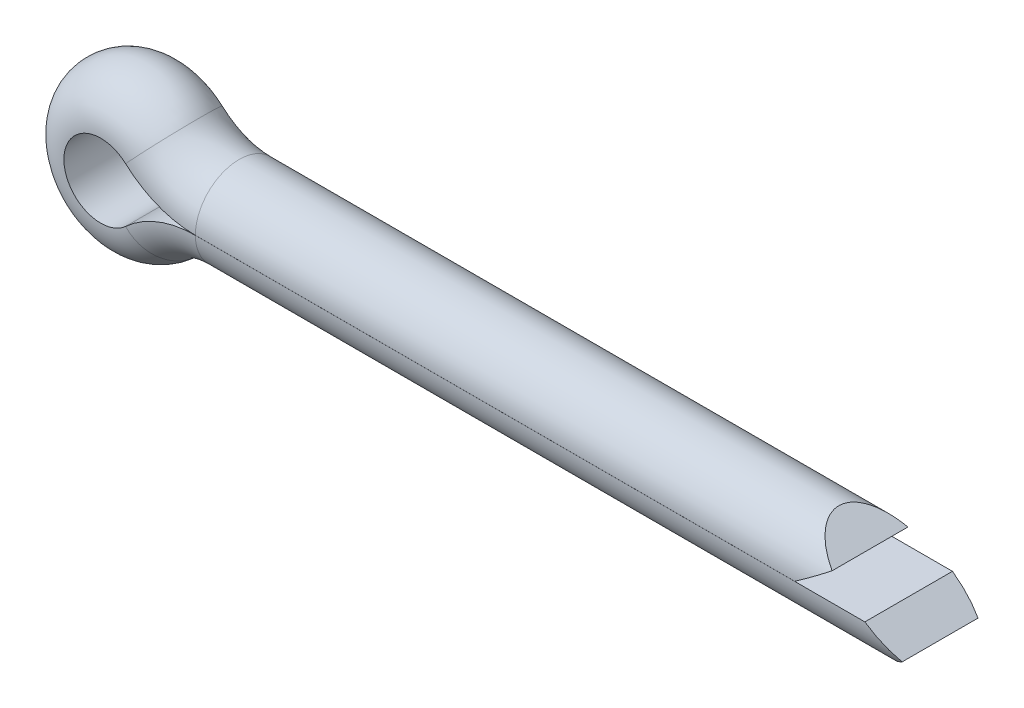
from build123d import *

# Parameters (mm, degrees)
CONECUT_DEPTH      = 41.341170006
CONECUT_DEPTH_BACK = 41.341170006


with BuildPart() as part:
    # Body: sweep along a path in Sketch2
    with BuildLine(Plane.XY) as body_path:
        Line((36, 2.5), (0, 2.5))
        ThreePointArc((0, 2.5), (-1.229728386, 2.730698436), (-2.292225201, 3.391420912))
        ThreePointArc((-2.292225201, 3.391420912), (-10, 0), (-2.292225201, -3.391420912))
        ThreePointArc((-2.292225201, -3.391420912), (-1.229728386, -2.730698436), (0, -2.5))
        Line((0, -2.5), (40, -2.5))
    # Sketch1 → Body (sweep)
    with BuildSketch(Plane(origin=(36, 0, 0), x_dir=(0, 0, -1), z_dir=(1, 0, 0))):
        with BuildLine():
            Line((-2.4999992, 0.002), (2.4999992, 0.002))
            ThreePointArc((2.4999992, 0.002), (0, 2.5), (-2.4999992, 0.002))
        make_face()
    sweep(path=body_path.line)

    # Sketch3 → ConeCut (cut, two sides: drawn at the far end of the back side and taken through both)
    with BuildSketch(Plane.XY.offset(-CONECUT_DEPTH_BACK)):
        Polygon((36, 1.251), (34.210475082, 2.51), (40.01, 2.51), (40.01, -2.51), (38.210475082, -2.51), (40, -1.251), (38.204873421, 0), (34.204873421, 0), align=None)
    extrude(amount=CONECUT_DEPTH + CONECUT_DEPTH_BACK, mode=Mode.SUBTRACT)


solid = part.part
